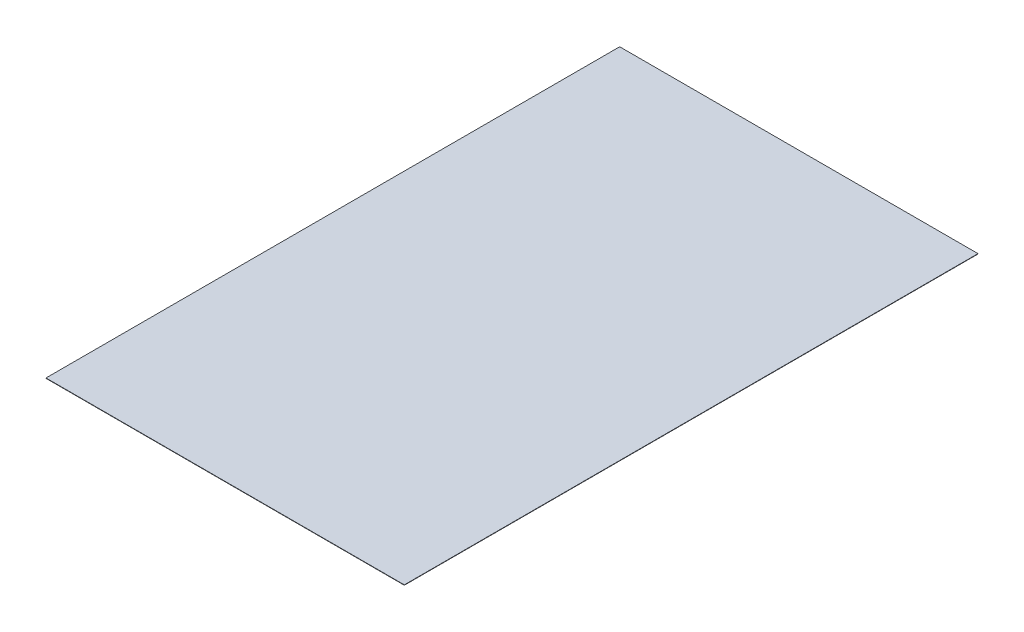
from build123d import *

# Parameters (mm, degrees)
SKETCH1_W           = 1000
SKETCH1_H           = 1601
BOSS_EXTRUDE1_DEPTH = 1


with BuildPart() as part:
    # Sketch1 → Boss-Extrude1 (new body)
    with BuildSketch(Plane(origin=(0, 0, 0), x_dir=(1, 0, 0), z_dir=(0, 1, 0))):
        Rectangle(SKETCH1_W, SKETCH1_H)
    extrude(amount=BOSS_EXTRUDE1_DEPTH)


solid = part.part
